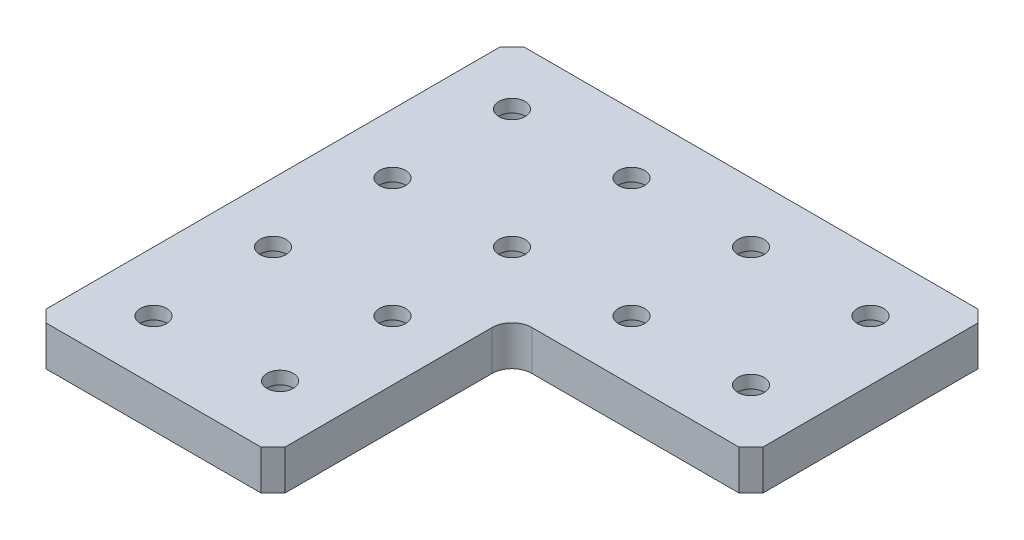
SolidWorks part; units mm, degrees
material "A6061 T6"
ref_plane "前视基准面" through (0, 0, 0) normal (0, 0, 1) x (1, 0, 0)
ref_plane "上视基准面" through (0, 0, 0) normal (0, 1, 0) x (1, 0, 0)
ref_plane "右视基准面" through (0, 0, 0) normal (1, 0, 0) x (0, 0, -1)
sketch "草图1" plane through (0, 0, 0) normal (0, 1, 0) x (1, 0, 0)
  line L1 (-60, 60) -> (60, 60)
  line L2 (-60, 60) -> (-60, -60)
  line L3 (-60, -60) -> (60, -60)
  line L4 (60, 60) -> (60, -60)
  line L5 (-60, 60) -> (60, -60) construction
  line L6 (-60, -60) -> (60, 60) construction
  point P0 (0, 0)
  dimension "D1" = 120
  dimension "D2" = 120
extrude "凸台-拉伸1" add sketch "草图1" along normal blind 10
sketch "草图2" plane through (0, 10, 0) normal (0, 1, 0) x (1, 0, 0)
  line L0 (60, 60) -> (-60, 60) construction
  line L1 (60, -60) -> (0, -60)
  line L2 (60, -60) -> (60, 0)
  line L3 (60, 0) -> (0, 0)
  line L4 (0, -60) -> (0, 0)
  line L5 (-60, 60) -> (-60, -60) construction
  dimension "D1" = 60
  dimension "D2" = 60
extrude "切除-拉伸1" cut sketch "草图2" against normal blind 25
chamfer "倒角1" distance 3 angle 45 5 edges at (60, 5, -60) (60, 5, 0) (0, 5, 60) (-60, 5, 60) (-60, 5, -60)
fillet "圆角1" radius 5 1 edges at (0, 5, 0)
hole_wizard "打孔尺寸(%根据)内六角圆柱头螺钉的类型1" positions "草图3" profile "草图4" counterbore size "M6" standard "GB"
sketch "草图3" plane through (0, 0, 0) normal (0, -1, 0) x (-1, 0, 0)
  line L0 (-57, 60) -> (57, 60) construction
  line L1 (60, 57) -> (60, -57) construction
  line L2 (57, -60) -> (3, -60) construction
  line L3 (-60, 3) -> (-60, 57) construction
  point P0 (45, 45)
  point P2 (45, 15)
  point P4 (15, 45)
  point P6 (15, 15)
  point P8 (-45, 45)
  point P10 (-45, 15)
  point P12 (45, -15)
  point P14 (45, -45)
  point P16 (15, -43.2239)
  point P18 (15, -15)
  point P30 (-15, 45)
  point P32 (-15, 15)
  dimension "D1" = 15
  dimension "D2" = 30
  dimension "D3" = 15
  dimension "D4" = 30
  dimension "D5" = 15
  dimension "D6" = 30
  dimension "D7" = 15
  dimension "D8" = 30
sketch "草图4" plane through (-45, 0, -45) normal (1, 0, 0) x (0, 0, -1)
  line L0 (0, 0) -> (0, 26.9828)
  line L1 (0, 26.9828) -> (3.3, 25)
  line L2 (3.3, 25) -> (3.3, 6.8)
  line L3 (3.3, 6.8) -> (5.5, 6.8)
  line L4 (5.5, 6.8) -> (5.5, 0)
  line L5 (5.5, 0) -> (0, 0)
  line L10 (0, 26.9828) -> (-3.3, 25) construction
  line L11 (0, -6.35) -> (0, 107.95) construction
  dimension "孔直径" = 6.6
  dimension "孔深度" = 25
  dimension "柱形沉头孔直径" = 11
  dimension "柱形沉头孔深度" = 6.8
  dimension "导头角度" = 118
